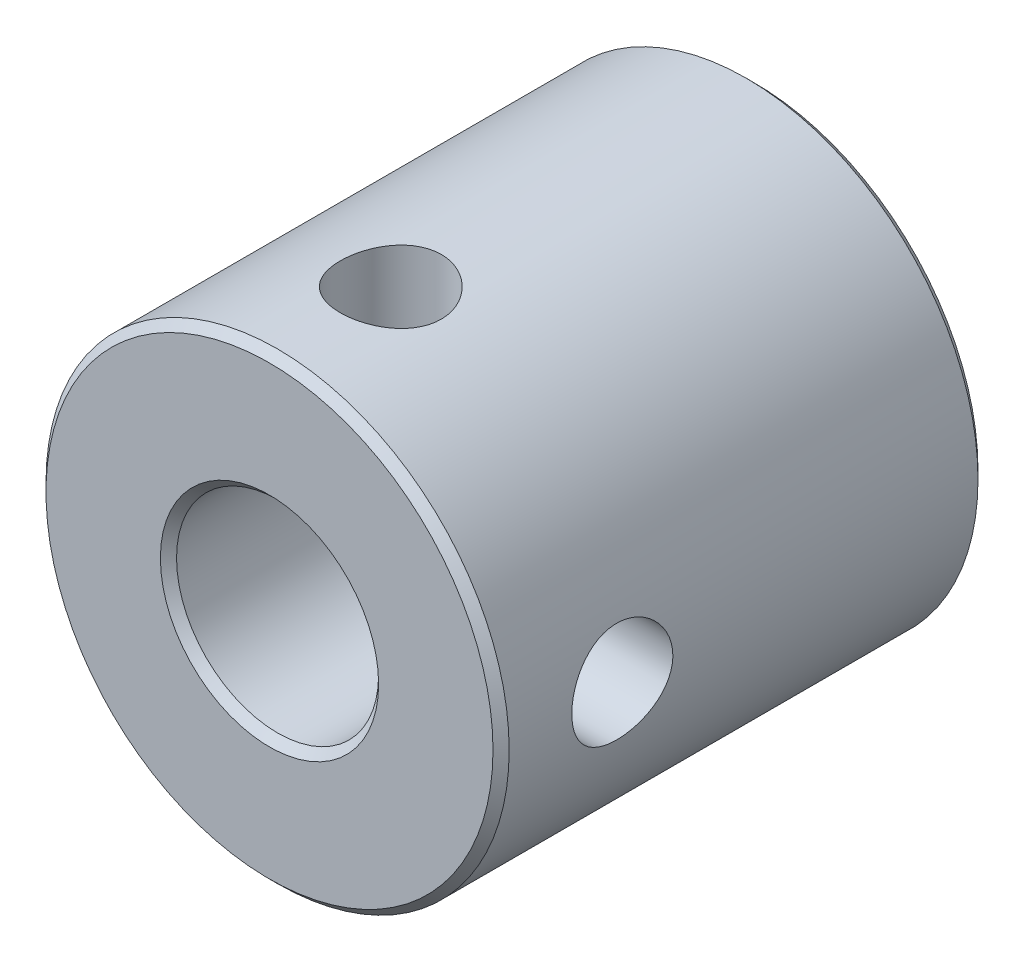
SolidWorks part; units mm, degrees
material "7075-T6"
ref_plane "Front Plane" through (0, 0, 0) normal (0, 0, 1) x (1, 0, 0)
ref_plane "Top Plane" through (0, 0, 0) normal (0, 1, 0) x (1, 0, 0)
ref_plane "Right Plane" through (0, 0, 0) normal (1, 0, 0) x (0, 0, -1)
sketch "Sketch1" plane through (0, 0, 0) normal (0, 1, 0) x (1, 0, 0)
  line L0 (0, 0) -> (0, 2.2625) construction
  line L1 (2.7, 0) -> (5.53, 0)
  line L2 (2.5, 0.2) -> (2.5, 11.8)
  line L3 (2.7, 12) -> (5.53, 12)
  line L4 (5.73, 0.2) -> (5.73, 11.8)
  line L5 (2.5, 11.8) -> (2.7, 12)
  line L6 (2.5, 0.2) -> (2.7, 0)
  line L7 (5.53, 0) -> (5.73, 0.2)
  line L8 (5.53, 12) -> (5.73, 11.8)
  point P0 (2.5, 0)
  point P1 (5.73, 12)
  point P2 (2.5, 12)
  point P3 (5.73, 0)
  dimension "D1" = 5
  dimension "D2" = 11.46
  dimension "D3" = 12
revolve "Revolve1" add sketch "Sketch1" angle 360 about L0
hole_wizard "M3 Tapped Hole1" positions "Sketch2" profile "Sketch3" tap size "M3" standard "GB"
sketch "Sketch2" plane through (0, 0, 0) normal (0, 1, 0) x (1, 0, 0)
  point P0 (0, 3)
  dimension "D1" = 3
sketch "Sketch3" plane through (0, 0, -3) normal (1, 0, 0) x (0, 0, -1)
  line L0 (0, 0) -> (0, 5.73)
  line L1 (0, 5.73) -> (1.25, 5.73)
  line L2 (1.25, 5.73) -> (1.25, 0)
  line L5 (1.25, 0) -> (0, 0)
  line L11 (0, -6.35) -> (0, 107.95) construction
  dimension "通孔螺纹孔钻头直径" = 2.5
  dimension "通孔螺纹孔钻头深度" = 5.73
cosmetic thread "Cosmetic Thread1"
hole_wizard "M3 Tapped Hole2" positions "Sketch4" profile "Sketch5" tap size "M3" standard "GB"
sketch "Sketch4" plane through (0, 0, 0) normal (1, 0, 0) x (0, 0, -1)
  point P0 (3, 0)
  dimension "D1" = 3
sketch "Sketch5" plane through (0, 0, -3) normal (0, 1, 0) x (0, 0, 1)
  line L0 (0, 0) -> (0, 5.73)
  line L1 (0, 5.73) -> (1.25, 5.73)
  line L2 (1.25, 5.73) -> (1.25, 0)
  line L5 (1.25, 0) -> (0, 0)
  line L11 (0, -6.35) -> (0, 107.95) construction
  dimension "通孔螺纹孔钻头直径" = 2.5
  dimension "通孔螺纹孔钻头深度" = 5.73
cosmetic thread "Cosmetic Thread2" parameters "D2"=3
